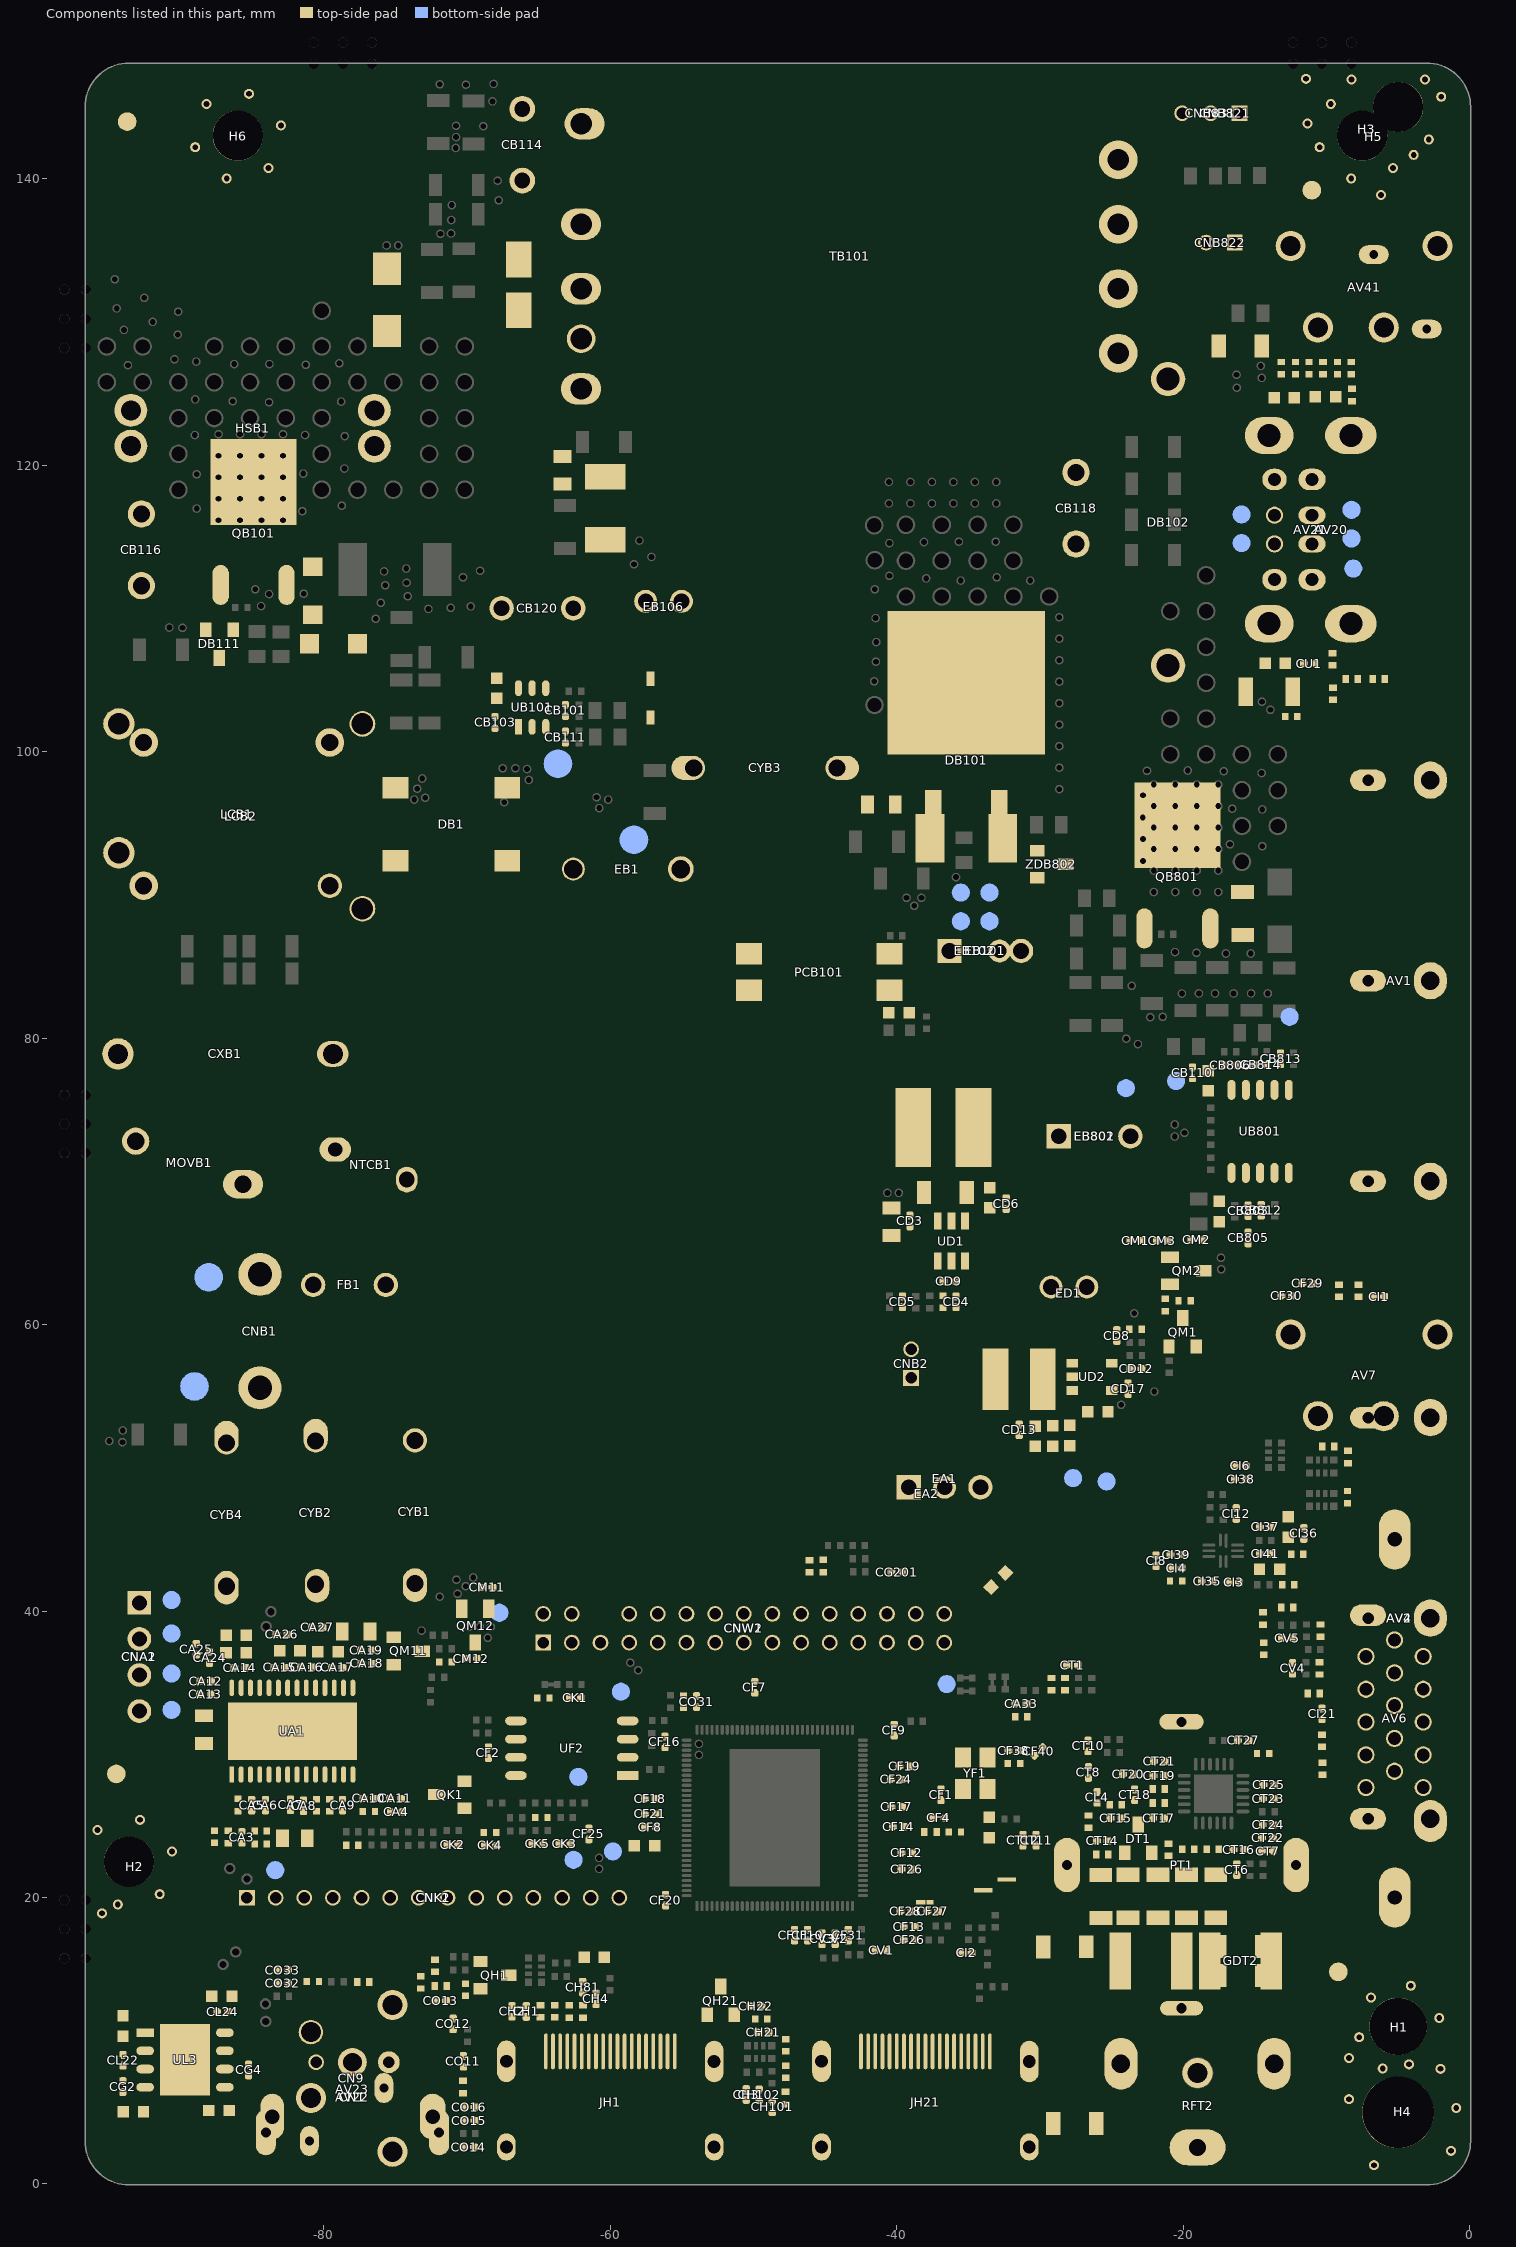
[diagram p0: the components of this part, seen from the top]
# Altium PCB MISC86372.PcbDoc (part 5 of 16)
Units mm, origin at the board's own origin, x right, y up, seen from the top; angles counter-clockwise.
Board outline 96.73 x 148.13 mm, 2 copper layers (TopLayer, BottomLayer), stack 1.571 mm thick; 578 components, 318 nets, 2702 pads, 836 vias.

## Footprints (in the part's own frame and the unit in brackets; to place one, negate y for a bottom-side part, rotate by r counter-clockwise, add the part's x,y. Pads: shape width x height; smd on the part's side, far side on the other; paste and mask are expansions set on the pad) (continued)
SIP2*15/2.0D-11 [mm] "浙江创佳；PHD-2*n-DK-6;,缺第6PIN；14.12.04"
  round 1.3 on Bottom Solder: 0(10,-1)
  rect 1.1x1.1 hole 0.8: 1(14,1)
  round 1.1 hole 0.8: 2(14,-1) 3(12,1) 4(12,-1) 5(10,1) 7(8,1) 8(8,-1) 9(6,1) 10(6,-1) 11(4,1) 12(4,-1) 13(2,1) 14(2,-1) 15(0,1) 16(0,-1) 17(-2,1) 18(-2,-1) 19(-4,1) 20(-4,-1) 21(-6,1) 22(-6,-1) 23(-8,1) 24(-8,-1) 25(-10,1) 26(-10,-1) 27(-12,1) 28(-12,-1) 29(-14,1) 30(-14,-1)
  rect 1.3x1.3 on Top Overlay: 372(14,1)
  round 1.3 on Top Overlay: 373(12,1) 374(-10,-1) 374(10,1) 375(8,1) 376(6,1) 377(4,1) 378(2,1) 379(0,1) 380(-2,1) 381(-4,1) 382(-6,1) 383(-8,1) 384(-10,1) 385(-12,1) 386(-14,1) 387(14,-1) 388(12,-1) 390(8,-1) 391(6,-1) 392(4,-1) 393(2,-1) 394(0,-1) 395(-2,-1) 396(-4,-1) 397(-6,-1) 398(-8,-1) 400(-12,-1) 401(-14,-1)
  silkscreen extent -16.07,-3.47 16.59,3.47
SIP2/2.0D-1 [mm] "捷仕泰/铭锋达"
  rect 1.3x1.3 on Top Overlay: 0(-1,0)
  round 1.3 on Top Overlay: 0(1,0)
  rect 1.1x1.1 hole 0.8: 1(-1,0)
  round 1.1 hole 0.8: 2(1,0)
  silkscreen extent -3,-3.2 3,1.8, body extent -3,-3.2 3,1.8, height 6
SIP2/2.0D-CP [mm] ";带扣插座与非带扣插座 兼容；15.07.11"
  rect 1.4x1.4 on Top Overlay: 0(-1,0)
  round 1.4 on Top Overlay: 0(1,0)
  rect 1.1x1.1 hole 0.8: 1(-1,0)
  round 1.1 hole 0.8: 2(1,0)
  silkscreen extent -3,-3.2 3,3.07, body extent -3,-3.2 3,1.8, height 6
SIP3/2.0D-CP [mm] "捷仕泰/铭锋达;带扣插座与非带扣插座 兼容；15.07.11"
  rect 1.4x1.4 on Top Overlay: 0(-2,0)
  round 1.4 on Top Overlay: 0(0,0) 0(2,0)
  rect 1.1x1.1 hole 0.8: 1(-2,0)
  round 1.1 hole 0.8: 2(0,0) 3(2,0)
  silkscreen extent -4,-3.2 4,3.07, body extent -4,-3.2 4,1.8, height 6
SIP4/2.5D-2 [mm] "捷仕泰，A2502-04-A5WA-P（为保证与SIP4/2.54D-1兼容。改PIN间距为2.52mm，18.05.28）"
  rect 1.905x1.905 on Top Overlay: 0(-3.78,0)
  round 1.905 on Top Overlay: 0(-1.26,0) 0(1.26,0) 0(3.78,0)
  rect 1.651x1.651 hole 1.05: 1(-3.78,0)
  round 1.651 hole 1.05: 2(-1.26,0) 3(1.26,0) 4(3.78,0)
  silkscreen extent -6.4,-3.6 6.4,3
SIP4/2.54D-1 [mm] "捷仕泰/铭锋达"
  rect 1.905x1.905 on Top Overlay: 0(-3.78,0)
  round 1.905 on Top Overlay: 0(-1.26,0) 0(1.26,0) 0(3.78,0)
  rect 1.651x1.651 hole 1.05: 1(-3.78,0)
  round 1.651 hole 1.05: 2(-1.26,0) 3(1.26,0) 4(3.78,0)
  silkscreen extent -6.44,-3.5 6.44,2.5, body extent -6.35,-3.5 6.35,2.5, height 7
SIP14/2.0D-1 [mm] "铭锋达/捷仕泰"
  rect 1.3x1.3 on Top Overlay: 0(-13,0)
  round 1.3 on Top Overlay: 0(-11,0) 0(-9,0) 0(-7,0) 0(-5,0) 0(-3,0) 0(-1,0) 0(1,0) 0(3,0) 0(5,0) 0(7,0) 0(9,0) 0(11,0) 0(13,0)
  rect 1.1x1.1 hole 0.8: 1(-13,0)
  round 1.1 hole 0.8: 2(-11,0) 3(-9,0) 4(-7,0) 5(-5,0) 6(-3,0) 7(-1,0) 8(1,0) 9(3,0) 10(5,0) 11(7,0) 12(9,0) 13(11,0) 14(13,0)
  silkscreen extent -15.12,-3.2 15.13,1.8, body extent -15,-3.2 15,1.8, height 6
SIP14/2.0D-5 [mm] "捷仕泰   A2004-14-A1MA-P,插线高度11mm"
  rect 1.3x1.3 on Top Overlay: 0(-13,0)
  round 1.3 on Top Overlay: 0(-11,0) 0(-9,0) 0(-7,0) 0(-5,0) 0(-3,0) 0(-1,0) 0(1,0) 0(3,0) 0(5,0) 0(7,0) 0(9,0) 0(11,0) 0(13,0)
  rect 1.1x1.1 hole 0.8: 1(-13,0)
  round 1.1 hole 0.8: 2(-11,0) 3(-9,0) 4(-7,0) 5(-5,0) 6(-3,0) 7(-1,0) 8(1,0) 9(3,0) 10(5,0) 11(7,0) 12(9,0) 13(11,0) 14(13,0)
  silkscreen extent -15,-2.13 15,3.07
SMD4532-1 [mm] "Brightking,4532-091-LF,气体放电管,雷电防护器件，17.06.12"
  rect 1.5x4 smd: 1(-2.15,0) 2(2.151,0)
  silkscreen extent -1.25,-1.79 1.23,1.71, body extent -2.41,-1.75 2.41,1.75, height 3
SMD4532-1-C1206 [mm] "Brightking,4532-091-LF,SMD4532-1兼容C1206封装，19.01.08"
  rect 1.6x1 smd paste-5 mask-5: 1(-1.016,-1.501) 1(1.016,-1.499) 2(-1.016,1.501) 2(1.016,1.501)
  rect 1.6x1 on Top Paste paste-5 mask-5: 1(-1.016,-1.501) 1(1.016,-1.501) 2(-1.016,1.501) 2(1.016,1.501)
  rect 4x1.5 smd paste-5 mask-5: 1(0,-2.15) 2(0,2.151)
  rect 4.001x0.903 on Top Paste: 1(0.05,-2.499) 2(0.05,2.499)
  silkscreen extent -1.96,-1.16 1.96,1.2, body extent -1.82,-2.41 1.81,2.41, height 3
SO-23 [mm] "双向二极管封装"
  rect 0.8x1 smd: 1(0.953,1.016) 3(-0.953,1.016)
  rect 0.8x1.1 smd: 2(0,-0.966)
  silkscreen extent -1.55,-0.86 1.55,0.36, body extent -1.5,-1.25 1.5,1.25, height 1.1
SOIC8 [mm] "W25X40BVSNIG/GD25Q32BSIG/GD25LQ16"
  rect 1.5x0.6 smd: 1(-3.9,1.905)
  oval 1.5x0.6 smd: 2(-3.9,0.635) 3(-3.9,-0.635) 4(-3.9,-1.905) 5(3.9,-1.905) 6(3.9,-0.635) 7(3.9,0.635) 8(3.9,1.905)
  silkscreen extent -4.37,-2.65 2.7,3.38, body extent -4.05,-2.69 4.05,2.69, height 2.17
SOP8/1.27-3 [mm] "LEADCHIP;LC1118;14-05-09"
  rect 1.238x0.6 smd: 1(-2.783,1.905)
  oval 1.238x0.6 smd: 2(-2.783,0.635) 3(-2.783,-0.635) 4(-2.783,-1.905) 5(2.783,-1.905) 6(2.783,-0.635) 7(2.783,0.635) 8(2.783,1.905)
  rect 3.5x5 smd paste-3 mask-3: EPAD(0,0)
  silkscreen extent -3.42,-2.5 4.16,3.42, body extent -3.1,-2.5 3.1,2.5, height 1.76
SOP10/1.0-1 [mm] "ON BRIGHT;OB3350X"
  oval 1.4x0.55 smd: 1(-2.9,2) 2(-2.9,1) 3(-2.9,0) 4(-2.9,-1) 5(-2.9,-2) 6(2.9,-2) 7(2.9,-1) 8(2.9,0) 9(2.9,1) 10(2.9,2)
  silkscreen extent -4.6,-2.55 2.05,2.55, body extent -2.05,-2.55 2.05,2.55, height 1.75
SOT-23 [mm]
  rect 0.8x1 smd: B(0.953,1.016) E(-0.953,1.016)
  rect 0.8x1.1 smd: C(-0.013,-0.966)
  silkscreen extent -1.55,-0.81 1.55,0.36, body extent -1.5,-1.25 1.5,1.25, height 1.1
SOT-23-1 [mm]
  rect 0.8x1.1 smd: D(0,-1.15)
  rect 0.8x1.27 smd: G(0.95,1.2) S(-0.95,1.2)
  TopLayer pour cut-out: -1.583,0.903 -1.583,-0.905 1.587,-0.905 1.587,0.903
  silkscreen extent -1.55,-1.05 1.55,0.33, body extent -1.52,-1.48 1.52,1.48, height 1.25
SOT-23-5 [mm] "LPW5206(1.295mm)"
  rect 0.6x0.8 smd: 1(-0.95,-1.375) 2(0,-1.375) 3(0.95,-1.375) 4(0.95,1.375) 5(-0.95,1.375)
  silkscreen extent -2.07,-1.63 1.5,0.85, body extent -1.5,-0.85 1.5,0.85, height 1.45
SOT-23-6 [mm] "RICHTEK RT9266//RT7295A(1mm)"
  rect 0.55x1.2 smd: 1(-0.95,-1.4) 2(0,-1.4) 3(0.95,-1.4) 4(0.95,1.4) 5(0,1.4) 6(-0.95,1.4)
  silkscreen extent -2.18,-1.82 1.55,0.9, body extent -1.55,-0.9 1.55,0.9, height 1.3
SOT-26 [mm] "LD7536R"
  rect 0.5x1.1 smd: 1(0.95,1.35)
  oval 0.5x1.1 smd: 2(0,1.35) 3(-0.95,1.35) 4(-0.95,-1.35) 5(0,-1.35) 6(0.95,-1.35)
  silkscreen extent -1.55,-2.54 1.55,2.9, body extent -1.55,-0.9 1.55,0.9, height 1.45
SSOP28/0.65-5 [mm] "TI;TPA3140D2PWPR;15.07.08"
  rect 1.15x0.34 smd: 1(-3.025,4.225)
  oval 1.15x0.34 smd: 2(-3.025,3.575) 3(-3.025,2.925) 4(-3.025,2.275) 5(-3.025,1.625) 6(-3.025,0.975) 7(-3.025,0.325) 8(-3.025,-0.325) 9(-3.025,-0.975) 10(-3.025,-1.625) 11(-3.025,-2.275) 12(-3.025,-2.925) 13(-3.025,-3.575) 14(-3.025,-4.225) 15(3.025,-4.225) 16(3.025,-3.575) 17(3.025,-2.925) 18(3.025,-2.275) 19(3.025,-1.625) 20(3.025,-0.975) 21(3.025,-0.325) 22(3.025,0.325) 23(3.025,0.975) 24(3.025,1.625) 25(3.025,2.275) 26(3.025,2.925) 27(3.025,3.575) 28(3.025,4.225)
  oct 1.05x1.318 on Top Paste mask+0.076: EPAD(-0.675,2.427) EPAD(-0.675,0.809) EPAD(-0.675,-0.809) EPAD(-0.675,-2.427) EPAD(0.675,2.427) EPAD(0.675,0.809) EPAD(0.675,-0.809) EPAD(0.675,-2.427)
  oct 1.05x1.318 on Top Solder mask+0.076: EPAD(-0.675,2.427) EPAD(-0.675,0.809) EPAD(-0.675,-0.809) EPAD(-0.675,-2.427) EPAD(0.675,2.427) EPAD(0.675,0.809) EPAD(0.675,-0.809) EPAD(0.675,-2.427)
  rect 4x9 smd paste-5 mask-5: EPAD(0,0)
  silkscreen extent -4.65,-4.9 4.64,5.32, body extent -2.25,-4.9 2.25,4.9, height 1.2
T-13.2×12.4×7.7-F14.5 [mm] "LHD;13.2×12.4×7.7-F14.5 中心出口高度6.3mm；160713(18.08.30 优化短槽孔）(19.03.11,优化地孔与IEC一致）"
  oval 2.5x3.8 on Top Overlay paste-4 mask-4: 0(-5.35,6.1) 0(5.35,6.1)
  oval 4.1x2.7 on Top Overlay paste-4 mask-4: 0(0,0.25)
  round 2.3 on Top Overlay: 0(0,5.45)
  round 2.1 hole 1.4: 1(0,5.45)
  oval 2.3x3.6 hole 1.3 slot 2.6 at 90 deg: 2(-5.35,6.1) 4(5.35,6.1)
  oval 3.9x2.5 hole 1.2 slot 2.6 at 0 deg: 3(0,0.25)
  KeepOutLayer pour cut-out: -1.438,5.45 -1.329,4.902 -1.019,4.438 -0.555,4.128 -0.007,4.019 -0.007,4.019 0.541,4.128 1.005,4.438 1.315,4.902 1.424,5.45 1.424,5.45 1.315,5.998 1.005,6.462 0.541,6.772 -0.007,6.881 -0.007,6.881 -0.555,6.772 -1.019,6.462 -1.329,5.998 -1.438,5.45
  silkscreen extent -6.3,0 6.3,7.9, body extent -7.55,-35.2 7.55,7.7, height 13.85
T/EQ2414*10 [mm] "SQ，SYEQ2414Z-T012064B(BLACK)，0114_2019"
  oval 3x2.4 on Top Overlay mask+0.076: 0(-21.5,-9.25) 0(-21.5,-5.75) 0(-21.5,-2.25) 0(-21.5,2.25) 0(-21.5,9.25)
  round 2.9 on Top Overlay mask+0.076: 0(16,-6.75) 0(16,-2.25) 0(16,2.25) 0(16,6.75)
  oval 2.8x2.2 hole 1.5 copper offset 0.25,0 mask+0.051: 1(-21.5,9.25)
  oval 2.8x2.2 hole 1.5 mask+0.051: 3(-21.5,2.25) 4(-21.5,-2.25) 6(-21.5,-9.25)
  round 2 / inner oval 2.8x2.2 / far side oval 2.8x2.2 hole 1.5 mask+0.051: 5(-21.5,-5.75)
  round 2.7 hole 1.5 mask+0.051: 7(16,-6.75) 8(16,-2.25) 9(16,2.25) 10(16,6.75)
  silkscreen extent -23,-12.75 17.5,12.75, body extent -20.35,-12.75 14.35,12.75, height 14.5
TO-252-GDS [mm] "SC08440  IRLR024N"
  rect 6x6 smd: D(0,0)
  oval 1.143x2.794 smd: G(-2.3,-7.2) S(2.3,-7.2)
  silkscreen extent -3.4,-5.64 3.4,3.4, body extent -3.4,-7.75 3.4,2.45, height 2.5
TP [mm] "TEST POINT"
  round 1.27 smd paste-1.27: 1(0,0)
TP-80 [mm] "TEST POINT;2mm"
  round 2 smd paste-1.27: 1(0,0)
TP-TDT [mm] "电源放电测试点，间隔7.5mm"
  round 2 smd paste-2: 1(-3.75,0) 2(3.75,0)
  silkscreen extent -5.75,-2 5.75,2
TP_BL [mm] "TEST POINT,专用背光测试点"
  round 1.27 smd paste-1.27: 1(0,0)
  silkscreen extent -6.4,-0.97 0.95,0.96
USB1-HD-2 [mm] "捷仕泰 ： U2504M-04-E1WD-C；170204加宽后壳丝印(18.03.12,更新信号脚孔径）"
  oval 2.7x3.9 on Top Overlay: 0(-6.57,10.257) 0(6.57,10.247)
  oval 1.7x2.1 on Top Overlay: 0(-3.5,12.957) 0(3.5,12.957)
  oval 1.5x1.9 hole 0.9 slot 1.4 at 90 deg: 1(-3.5,12.957) 4(3.5,12.957)
  oval 1.4x2.1 on Top Overlay: 1(-1,12.957) 2(1,12.957)
  oval 1.2x1.9 hole 0.9 slot 1.4 at 90 deg: 2(-1,12.957) 3(1,12.957)
  oval 2.4x3.6 / inner oval 2.4x3.6 / far side oval 2.8x4 hole 1.6 slot 2.3 at 90 deg: 5(6.57,10.247) 6(-6.57,10.247)
  TopLayer pour cut-out: 2.433,14.667 4.428,14.667 4.532,14.647 4.62,14.588 4.678,14.5 4.699,14.396 4.699,14.396 4.699,11.335 4.68,11.238 4.625,11.156 4.542,11.101 4.445,11.081 4.445,11.081 2.422,11.081 2.422,14.656
  KeepOutLayer pour cut-out: -3.49,14.696 -4.146,14.566 -4.703,14.194 -5.075,13.637 -5.206,12.98 -5.206,12.98 -5.206,12.94 -5.068,12.25 -4.677,11.665 -4.092,11.275 -3.402,11.137 -3.402,11.137 2.42,11.137 2.637,11.18 2.821,11.303 2.943,11.487 2.986,11.703 2.986,11.703 2.986,14.149 2.944,14.361 2.824,14.541 2.644,14.661 2.432,14.704 2.432,14.704 -3.482,14.704 -3.485,14.703 -3.487,14.701 -3.489,14.699 -3.49,14.696
  silkscreen extent -7.1,2.04 7.05,14.58, body extent -10,-87.25 10,14.14, height 8.2
USB2-HD-1 [mm] "双盟 DUAL USB A/F 90°,20170921修改宽度到15.2mm"
  oval 2.9x3.7 on Top Overlay: 0(-6.57,16) 0(-6.57,10.3) 0(6.57,16) 0(6.57,10.3)
  round 1.85 on Top Overlay: 0(-3.5,13.01) 0(-3.5,15.63) 0(3.5,13.01) 0(3.5,15.63)
  round 1.4 on Top Overlay: 0(-1,15.63) 0(-1,13.01) 0(1,15.63) 0(1,13.01)
  oval 1.5x1.7 hole 0.9: 1(-3.5,15.63) 4(3.5,15.63) 5(-3.5,13.01) 8(3.5,13.01)
  round 1.2 hole 0.9: 2(-1,15.63) 3(1,15.63) 6(-1,13.01) 7(1,13.01)
  oval 2.6x3.4 hole 1.6 slot 2.3 at 90 deg: 9(-6.57,16) 10(6.57,16) 11(-6.57,10.3) 12(6.57,10.3)
  KeepOutLayer pour cut-out: -5.206,13.033 -5.206,15.649 -4.578,15.021 -4.578,13.669 -5.214,13.033
  KeepOutLayer pour cut-out: -3.49,14.749 -4.146,14.618 -4.703,14.246 -5.075,13.69 -5.206,13.033 -5.206,13.033 -5.206,12.993 -5.068,12.303 -4.677,11.718 -4.092,11.327 -3.402,11.19 -3.402,11.19 2.42,11.19 2.637,11.233 2.821,11.356 2.943,11.539 2.986,11.756 2.986,11.756 2.986,14.202 2.944,14.414 2.824,14.594 2.644,14.714 2.432,14.756 2.432,14.756 -3.482,14.756 -3.485,14.756 -3.487,14.754 -3.489,14.752 -3.49,14.749
  KeepOutLayer pour cut-out: -3.49,17.369 -4.146,17.238 -4.703,16.866 -5.075,16.31 -5.206,15.653 -5.206,15.653 -5.206,15.613 -5.068,14.923 -4.677,14.338 -4.092,13.947 -3.402,13.81 -3.402,13.81 2.42,13.81 2.637,13.853 2.821,13.976 2.943,14.159 2.986,14.376 2.986,14.376 2.986,16.822 2.944,17.034 2.824,17.214 2.644,17.334 2.432,17.376 2.432,17.376 -3.482,17.376 -3.485,17.376 -3.487,17.374 -3.489,17.372 -3.49,17.369
  silkscreen extent -6.7,2 6.7,17.25, body extent -7.5,0 7.5,17, height 16.1
VR(13*5)-V-7.5 [mm] "为勤,VARISTOR,17.01.04修改为椭圆孔;160105更新椭圆孔"
  oval 2.8x2 hole 1.2 slot 2 at 0 deg: 1(3.75,-1.5)
  round 1.9 hole 1.2: 2(-3.75,1.5)
  round 2.1 on Top Overlay: 2(-3.75,1.5)
  oval 3x2.2 on Top Overlay: 2(3.75,-1.5)
  silkscreen extent -6.65,-2.5 6.42,2.5, body extent -6.5,-2.75 6.5,2.75, height 15.5
XTAL-S-3 [mm] "三星（SQ3D03200D2IBA）晶振"
  rect 1.4x1.1 smd: 1(-1.1,-0.85) 2(1.1,-0.85) 3(1.1,0.85) 4(-1.1,0.85)
  silkscreen extent -2.37,-1.91 1.65,1.3, body extent -1.65,-1.3 1.65,1.3, height 0.8

## Part data
5V DM0 DM1 DP0 DP1 LOUT+ LOUT- PWM_REF ROUT+ ROUT- RXD TP_12VA+ TP_12VA- TP_12VB+ TP_12VB- TP_L TP_LED+ TP_LED- TP_N TXD UART_RX UART_TX: library part TEST
AV1 AV2: library part "RCA端子,RCA Jack,AV3,H,Yellow、White、Red,CH5.5,D14,Seal,DIP,RC075-F03L3BY-A,YUQIU-DLMI-AV", "CN-AV-D14-#-#"
AV4: library part "RCA端子,RCA Jack,AV3,H,Green、Blue、Red,CH5.5,D14,Seal,DIP,RC075-F03L3BY-B,YUQIU-DLMI-YPbPr", "CN-YPbPr-D14-#-#"
AV6: library part WLHD-051A-DLMI-DB15, "CN-DB15-horizontal-#-#-#"
AV7: library part "耳机端子,Earphone  Jack,H,Φ3.5,CH7.0,Black,Seal,SMD,PJ7723-F03L3BE-C,YUQIU-DLMI", "CN-headphone"
AV20: library part XXX.XXX.0002687, "USB jack,USB Jack,H,Single,flange,DIP,103411271,VAST-DLMI"
AV21: library part XXX.XXX.0001070-DLMI, "USB jack,USB Jack,H,Double,Black,flange,DIP,WLUS-074B,WLCO-DLMI"
AV22: library part "RCA端子,RCA Jack,AV1,H,Orange,CH5.5,Seal,DIP,AV38A-01S-5020,QS-DLMI"
AV23: library part 光纤端子,OPTICAL,H,DIP,GQ-03-08C1,QS-DLMI, "CN-DLMI-optical fibre"
AV41 CN9: library part XXX.XXX.0002138, "Earphone jack,Earphone Jack,H,Φ3.5,CH7.0,Black,switch,Seal,DIP,PJ7724-F05L3BY-D,YUQIU-DLMI"
BA1 BA2 BA3 BA4: library part 004.004.0000104-D, "Multilayer inductor,HF Inductor,220nH,±5%,0603,SMD,SWI0603F-R22J,Tai-tech-D"
BB101: library part 磁珠,BEAD,50ohm,3.0×4.0,9A,SMD,TP,SMB-302540-K5B-L1,SOLDIER-D
CA1 CA2 CD2: library part 004.003.0000386-D, "Ceramic capacitor,CAP MC,16V,10uF,±20%,X5R,0805,SMD,TP-D"
CA3 CA4: library part 004.003.0000549-D, "Ceramic capacitor,CAP MC,50V,3300pF,±10%,X7R,0402,SMD,TP-D"
CA5 CA6 CA10 CA11 CA14 CA15 CA16 CA17: library part 004.003.0000398-D, "Ceramic capacitor,CAP MC,16V,0.22uF,±20%,X5R,0402,SMD,TP-D"
CA7 CA9: library part 004.003.0000402-D, "Ceramic capacitor,CAP MC,16V,1uF,±20%,X5R,0402,SMD,TP-D"
CA8 CA12 CA18 CD3 CD4 CD6 CD8 CD9 CM1 CM2 CO32 CT1 CT11 CT12 CT17: library part 004.003.0000403-D, "Ceramic capacitor,CAP MC,16V,0.1uF,±20%,X5R,0402,SMD,TP-D"
CA13 CA19: library part 004.003.0000503-D, "Ceramic capacitor,CAP MC,50V,1000pF,±10%,X7R,0402,SMD,TP-D"
CA24 CA25 CA26 CA27: library part 004.003.0000534-D, "Ceramic capacitor,CAP MC,50V,2200pF,±10%,X7R,0402,SMD,TP-D"
CA31 CA32 CD7 CG1 CG3 CL3 CL21 CL23: library part 004.003.0000383-D, "Ceramic capacitor,CAP MC,6.3V,10uF,±20%,X5R,0603,SMD,TP-D"
CA33 CI12 CI37 CI38 CI39 CO12 CO15: library part 004.003.0000361-D, "Ceramic capacitor,CAP MC,6.3V,0.47uF,±10%,X5R,0402,SMD,TP-D"
CB101 CB803 CB814: library part 100pF-0402-NPO-±5%-50V-D
CB102 CB109 CB139: library part 0.1uF-0603-X7R-±10%-50V-D, "CAP"
CB103 CF29 CF30 CI35 CO11 CO13 CO14 CO16 CT18: library part 1000pF-0402-X7R-±10%-50V-D
CB110 CB806: library part 1000pF-0402-X7R-±10%-50V-D, "CAP"
CB111: library part 004.003.0000501-D, "Ceramic capacitor,CAP MC,50V,100pF,±5%,NPO,0402,SMD,TP-D"
CB114: library part C242G472J20A201(编带/法拉)-DAI, "CAP"
CB116: library part 004.003.0001895-DHAI, "Ceramic capacitor,CAP CD,2KV,100pF,±5%,SL,OK,5.0mm,DIP,TP,TDK-DHAI"
CB117 CB119: library part 1000pF-0805-NPO-±10%-200V-D, "CAP"
CB118: library part 004.003.0001892-DHAI, "Ceramic capacitor,CAP CD,1KV,220pF,±5%,SL,OK,5.0mm,DIP,TP,TDK-DHAI"
CB120: library part 004.003.0001665, "Ceramic capacitor,CAP CD,1KV,4700pF,±20%,Y5U,K,5.0mm,DIP,TP,Walsin-DHAI"
CB129 CB808: library part 22pF-1206-NPO±5%-1000V-D
CB801: library part 1uf-0603-X7R-±10%-25V-D
CB805: library part 0.1uF-0402-X7R-±10%-16V-D
CB812: library part 0.033uF-0402-X7R-±10%-16V-D
CB813: library part 4700pF-0402-X7R-±10%-50V-D
CD1: library part 10uF-1206-X5R-±10%-16V-D
CD5: library part 004.003.0000570-D, "Ceramic capacitor,CAP MC,50V,56pF,±5%,NPO,0402,SMD,TP-D"
CD10 CD14 CD15 CD16 CF3 CF5 CF15 CI9 CI40 CU2: library part 10uF-0603-X5R-±20%-6.3V-D
CD12: library part 3300pF-0402-X7R-±10%-50V-D
CD13 CD17 CH1 CH2 CH21 CH22 CI36 CI41 CK2 CK4 CK5 CM11 CT19 CT21 CT22 CT25: library part 0.1uF-0402-X5R-±20%-16V-D
CD101 CD102 DA31 DA32 DA33 DI6 DK1 DK2 DK3 DO1 DV1 DV2 DV3 DV4 DV5 DV6 DV7 DV8 DV9: library part AVLC18S02003-D
CF1 CF4: library part 004.003.0000527-D, "Ceramic capacitor,CAP MC,50V,18pF,±5%,NPO,0402,SMD,TP-D"
CF2 CF7 CF8 CF9 CF10 CF12 CF13 CF14 CF17 CF27 CG201 CI3 CI4 CI6 CI8 CT27: library part 0.1uF-0402-Y5V-+80%-20%-16V-D
CF11 CF16 CF18 CF19 CF20 CF21 CF25 CF28 CG4 CH81 CL24 CU1: library part 1uF-0402-X5R-±20%-6.3V-D
CF24 CG2 CL22: library part 004.003.0000100-D, "Ceramic capacitor,CAP MC,6.3V,2.2uF,±20%,X5R,0402,SMD,TP-D"
CF26 CF31 CI2 CT16 CV1 CV2 CV3: library part 0.047uF-0402-X7R-±10%-16V-D
CF38 CF40 CV4 CV5: library part 30pF-0402-NPO-±5%-50V-D
CH3 CH4 CT6 CT7: library part 004.003.0000530-D, "Ceramic capacitor,CAP MC,50V,22pF,±5%,NPO,0402,SMD,TP-D"
CH101 CH102: library part 220pF-0402-X7R-±10%-50V-D
CI1 CI21: library part 10pF-0402-NPO-±5%-50V-D
CK1: library part 22pF-0402-NPO-±5%-50V-D
CK3: library part 004.003.0000506-D, "Ceramic capacitor,CAP MC,50V,0.01uF,±10%,X7R,0402,SMD,TP-D"
CL4: library part 004.003.0000382-D, "Ceramic capacitor,CAP MC,6.3V,1uF,±20%,X5R,0402,SMD,TP-D"
CM3 CM12 CT20 CT26: library part 0.022uF-0402-X7R-±10%-16V-D
CN1: library part "RCA端子,RCA Jack,AV1,H,Yellow,CH5.5,Seal,DIP,AV38A-01S-5030,QS-DLMI"
CNA1: library part XXX.XXX.0000595-DHMI, "Connector socket,connect jack,4Pin,D2.50,D,L=2.8mm,DIP,CNJST-DHMI"
CNA2: library part XXX.XXX.0000676-DHMI, "Connector socket,connect jack,4Pin,D2.54,D,SNAP,L=3.0mm,DIP,BOOM-DHMI"
CNB1: library part "连接插座,connect jack,2Pin,D7.92,L,SNAP,Fool-proofing,nature,L=2.8mm,DIP,AMA-DLMI", "AC socket"
CNB2 CNB821 CNB822: library part XXX.XXX.0001753, "Connector socket,connect jack,2Pin,D2.0,D,L=2.8mm,DIP,AMA-DHMI"
CNB831: library part XXX.XXX.0001754, "Connector socket,connect jack,3Pin,D2.0,D,L=2.8mm,DIP,AMA-DHMI"
CNK1: library part 14PIN-2.0-D-H-G-带扣-J-DHMI
CNK2: library part 14PIN-2.0-D-H-G-DHMI
CNW1: library part "连接插座,connect jack,2×15Pin/without pin6,D2.0,D,SNAP,Fool-proofing,Nature,L=2.6mm,DIP,CJ", "CN-latched"
CNW2: library part 2×15PIN-2.0-D-H-M(脚长=2.6mm)(缺6PIN)-LK-DHMI, "CN-straight gold pin"
CO31: library part 33pF-0402-NPO-±5%-50V-D
CO33 CT23: library part 330pF-0402-NPO-±5%-50V-D
"Conformal Coating": library part 三防漆,25kg/Can,Peters
CT8 CT10: library part 004.003.0000556-D, "Ceramic capacitor,CAP MC,50V,47pF,±5%,NPO,0402,SMD,TP-D"
CT13: library part 0.47uF-1206-Y5V-+80%-20%-16V-D
CT14: library part 220pF-0402-NPO-±5%-50V-D
CT15: library part 180pF-0402-NPO-±5%-50V-D
CT24: library part 6800pF-0402-X7R-±10%-50V-D
CT41 CT43 CT44 CT45 CT47 CT48: library part 1000pF-1206-X7R-±20%-2000V-D
CT42 CT46: library part 1000pF-1206-X7R±10%-2000V-D
CXB1: library part "X电容,CAP X2,MP,275VAC,0.47uF,±10%,S,15mm-Mini,PC,DIP,BM-DHMI", "CAP"
CYB1 CYB2 CYB3 CYB4: library part "Y电容,CAP Y1,CD,470pF,400VAC,±20%,KS,10mm,Y5U,DIP,Walsin-DHMI", "Y1 capacitor"
DB1: library part 004.005.0000860-D, "Bridge rectifier,DIO BRD,3A,800V,YBS,SMD,YBS3010A,YJ-D"
DB101: library part MBRB10150CT(GOOD-ARK)-D, "Diode"
DB102: library part 004.005.0000308, "Rectifier diode,DIO UFRD S,4A,800V,DO-201AD,DIP,MUR480ERLG,ON-DLMI"
DB104: library part M7(WEJ)-D, "Diode"
DB106: library part 004.005.0000504-D, "Rectifier diode,DIO FRD S,2A,800V,DO-214AC,SMD,GR2KA,GOOD-ARK-D"
DB107: library part BAV21WS-D, "Diode"
DB109 DB110: library part "整流二极管,DIO FRD S,1.2A,800V,eSGA,SMD,R12K,GOOD-ARK-D"
DB111: library part LBAV70LT1G(LRC)-D, "Diode"
DH1 DH2 DH3 DH21 DH22 DH23 DH81: library part 004.005.0000315-D, "TVS diode,DIO ESD,2.5pF,200V,0402,SMD,SFI0402-240E-2R5PP-LF,SFI-D"
DI1 DI2 DI3: library part AIES12U020R2-D
DI8 DI9: library part SFI0402-240E-2R5PP-LF-D
DT1: library part 004.005.0000195-D, "Switching diode,DIO SW D2,200mA,70V,SOT-23,SMD,BAV99,BLUE ROCKET-D"
DU1 DU2 DU3 DU4: library part 004.005.0000203-D, "TVS diode,DIO ESD,0.2pF,25V,0402,SMD,AIES12U020R2,AMOTECH-D"
EA1: library part 004.003.0000601-DHAI, "Aluminium electrolytic capacitor,CAP AL,16V,470uF,±20%,RK,P,5.0mm,10×12,DIP,TP,XL-DHAI"
EA2: library part 004.003.0000158-DHAI, "Aluminium electrolytic capacitor,CAP AL,16V,220uF,±20%,LD,KF,P,2.5mm,6.3×11,DIP,TP,CapXon-DHAI"
EB1: library part "铝电解电容,CAP AL,450V,68uF,±20%,KM,BK,7.5mm,18×31.5,DIP,CapXon-DLMI", "CAP"
EB101: library part 470uF-25V-±20%-10×12.5-105℃-GF-编带-F=5.0(CapXon)-DHAI, "Electrolytic"
EB102: library part 270uF-16V-±20%-8×11.5-105℃-PS-短脚-F=3.5(Capxon), "Solid-state"
EB106: library part 10uF-50V-±20%-5×11-105℃-GH-编带-F=2.5(CapXon)-DHAI, "Electrolytic"
EB801: library part 004.003.0000876, "Aluminium electrolytic capacitor,CAP AL,100V,47uF,±20%,LD,SK,P,5.0mm,10×12.5,DIP,TP,Samxon-DHAI"
EB802: library part 004.003.0000945, "Aluminium electrolytic capacitor,CAP AL,160V,39uF,±20%,LD,DV,P,5.0mm,12.5×12,DIP,TP,Elite-DHAI"
ED1: library part 470uF-10V-±20%-6.3×11-105℃-黑底白字-编带-F=2.5-XF-DHAI, "Electrolytic"
EVA1 EVA2 EVA3 EVA4 EVA5 EVA6: library part 7×7×3mm-C-4305防火泡棉-黑色-DLMI, "EVA"
FB1: library part 004.026.0000010-DHMI, "Slow-blow fuse,FUSE T,P,3.15A,250VAC,8.5×4.0×8mm,DIP,TP,Walter-DHMI"
FU1: library part 004.026.0000039-D, "Self-recovering fuse,FUSE PTC,1.1A,6V,1206,SMD,TP,TLC-D"
GD1 GD2 GD3: library part 7.00×8.35mm-尼龙-白色-WQM-DHMI, "Mylar standoff"
GDT1: library part 004.005.0000675, "Gas discharge tube,GDT,700V,2000A,TP,4.5*3.2mm,SMD,4532-091-LF,Brightking-D"
GDT2: library part 004.005.0000675-C1206, "Gas discharge tube,GDT,700V,2000A,TP,4.5*3.2mm,SMD,4532-091-LF,Brightking-D"
GL1: library part 005.002.0000011, "Silicone,0.2g,general,60,white,SLD-8854W,XY-DHMI"
H1 H2 H3 H4 H5 H6: library part "Location hole-D"
HS1: library part 14×14×06-THD-HS, "SMD heatsink"
HSB1: library part 004.040.0006600-DHMI, "Heatsink,17.5×14.5×0.5mm,red copper sheet,matte tin plated,natural,four pins,WT-DHMI"
JH1 JH21: library part XXX.XXX.0001122-D, "HDMI jack,HDMI Jack,H,SMD,161031041(hull-SPCC ),VAST-D"
L3: library part FCM1005KF-121T06(120ohm-500mA)-D
L6 RI4 RO2 RO3 RT1 RU4: library part 004.002.0000558-D, "Thick-film resistor,RES,1/16W,0ohm,±5%,0402,SMD-D"
LCB1: library part SYUU10.5-L002-JM-DHMI, "Common-mode choke"
LCB2: library part "共模电感,Common Choke,UC15,10.5mH,0.13×1.0mm,48Ts,H14.0MAX,SYUC15-L10.5mA,DIP,UENO-DLMI", "Common-mode choke"
LD1: library part 004.004.0000017-D, "Power inductor,Power Inductor,4.7uH,±20%,2.8A,0.35×1P,DR5.8×4.5,SMD,SCD54TL-4R7M,Soldier-D"
LD2: library part SLN43T-6R8M-D
LF6 RA4 RA5: library part GND
LT2: library part SDCL1005CR27JTDF(顺络)-D
LT3 LT6 LT10: library part 004.004.0000087-D, "Multilayer inductor,HF Inductor,180nH,±5%,0402,SMD,SDCL1005CR18JTDF,Sunlord-D"
LT4 LT5: library part GZ1005U102CTF(1000ohm-300mA)-D
LT8: library part SDCL1005C68NJTDF(68nH-0402±5%-C)-D
LT9: library part 1Kohm-0402-±25%-D
M1 M2 M3 M4: library part MARK-D
ML1: library part MALAY
MOVB1: library part TVR10561KSW(为勤)-DHMI, "Varistor"
NTCB1: library part SCK102R55AMBY502(短脚/为勤)-DHMI, "Thermistor"
PCB101: library part LTV-817S-TA-B(光宝)-DMI, "Optocoupler"
PT1: library part 004.040.0000768-DMI, "Shield can,tinplate,natural,20.3×16.3×6mm,with sealed opening,LHD-DMI"
QB101: library part 场效应管,NMOS,5.2,650V,1.02ohm@ID=2.6A@VGS=10V,DPAK,TK5P65W,TOSHIBA-D, "N Channel Single MOSFET"
QB801: library part ME15N10(松木)-D, "N Channel Single MOSFET"
QH1 QH21 QM1: library part 004.006.0000007-D, "General transistor,Dynatron,NPN,0.2A,40V,60-300,SOT-23,KMBT3904,KEXIN-D"
QK1 QM11: library part LMBT3904LT1G-D-NPN, "Q-NPN-#-#-#"
QM2: library part 004.007.0000286-D, "Field-effect transistor,PMOS,-4.7A,-20V,70mohm@ID=-4.7A@VGS=-4.5V,SOT23-LC,LPB3443LT1G,LRC-D"
QM12: library part WPM3407C-3/TR-D
RA1 RA2 RM3: library part 004.002.0000689-D, "Thick-film resistor,RES,1/16W,4.7Kohm,±5%,0402,SMD-D"
RA3 RA14: library part 004.002.0000572-D, "Thick-film resistor,RES,1/16W,1Kohm,±5%,0402,SMD-D"
RA8 RD1 RD7 RM4: library part 004.002.0000579-D, "Thick-film resistor,RES,1/16W,100Kohm,±5%,0402,SMD-D"
RA9: library part 004.002.0000691-D, "Thick-film resistor,RES,1/16W,47Kohm,±5%,0402,SMD-D"
RA10: library part 004.002.0000575-D, "Thick-film resistor,RES,1/16W,10Kohm,±1%,0402,SMD-D"
RA11: library part 004.002.0000602-D, "Thick-film resistor,RES,1/16W,15Kohm,±1%,0402,SMD-D"
RA25: library part 004.002.0000562-D, "Thick-film resistor,RES,1/8W,10ohm,±5%,0805,SMD-D"
RA31 RA32 RF24 RH3 RH23 RI3 RI42 RI43 RK2 RK4 RK10: library part 1Kohm-0402-±5%-1/16W-D
RA33 RA34 RO21: library part 004.002.0000609-D, "Thick-film resistor,RES,1/16W,180ohm,±5%,0402,SMD-D"
RA35 RM14: library part 47Kohm-0402-±5%-1/16W-D